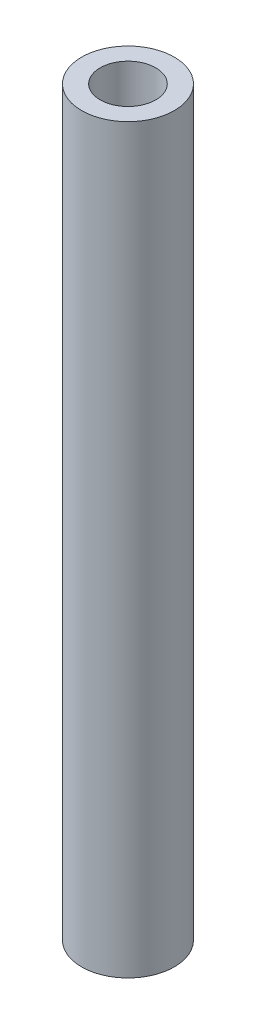
SolidWorks part; units mm, degrees
material "6061 合金"
ref_plane "前视基准面" through (0, 0, 0) normal (0, 0, 1) x (1, 0, 0)
ref_plane "上视基准面" through (0, 0, 0) normal (0, 1, 0) x (1, 0, 0)
ref_plane "右视基准面" through (0, 0, 0) normal (1, 0, 0) x (0, 0, -1)
other "Configuration Table"
sketch "草图1" plane through (0, 0, 0) normal (0, 1, 0) x (1, 0, 0)
  circle A0 centre (0, 0) radius 1.5
  circle A1 centre (0, 0) radius 2.5
  dimension "D1" = 3
  dimension "D2" = 5
extrude "凸台-拉伸1" add sketch "草图1" along normal blind 40
